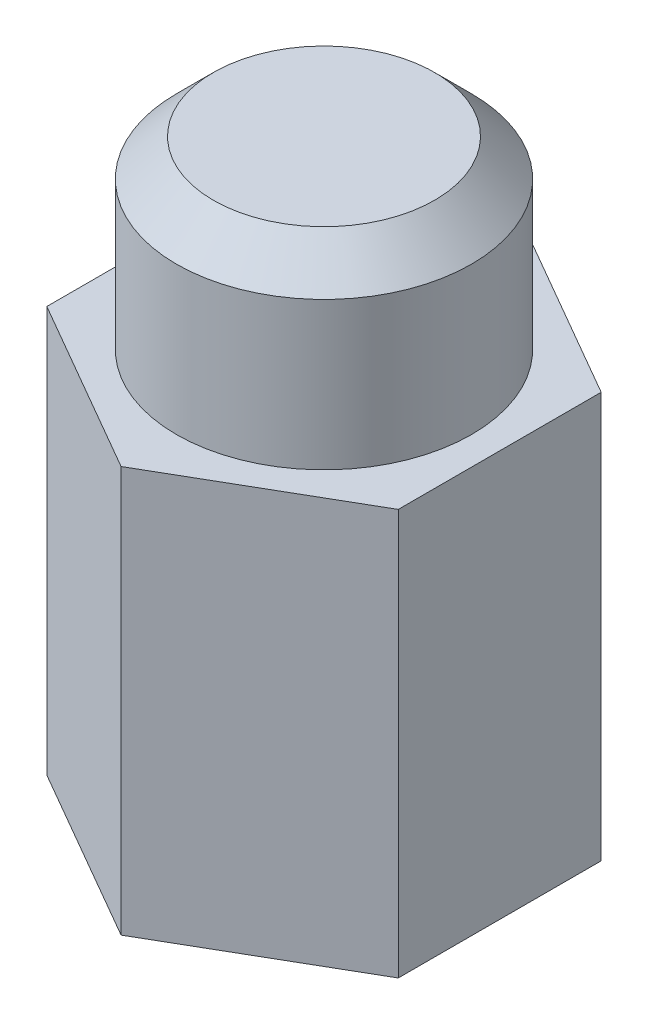
SolidWorks part; units mm, degrees
ref_plane "Front Plane" through (0, 0, 0) normal (0, 0, 1) x (1, 0, 0)
ref_plane "Top Plane" through (0, 0, 0) normal (0, 1, 0) x (1, 0, 0)
ref_plane "Right Plane" through (0, 0, 0) normal (1, 0, 0) x (0, 0, -1)
sketch "Sketch1" plane through (0, 0, 0) normal (0, 1, 0) x (1, 0, 0)
  line L1 (0, 5.5) -> (-4.7631, 2.75)
  line L2 (-4.7631, 2.75) -> (-4.7631, -2.75)
  line L3 (-4.7631, -2.75) -> (0, -5.5)
  line L4 (0, -5.5) -> (4.7631, -2.75)
  line L5 (4.7631, -2.75) -> (4.7631, 2.75)
  line L6 (4.7631, 2.75) -> (0, 5.5)
  circle A0 centre (0, 0) radius 4.7631 construction
  dimension "D1" = 11
extrude "Boss-Extrude1" add sketch "Sketch1" along normal mid plane 11
sketch "Sketch3" plane through (0, 5.5, 0) normal (0, 1, 0) x (1, 0, 0)
  circle A0 centre (0, 0) radius 4
  dimension "D1" = 8
extrude "Boss-Extrude2" add sketch "Sketch3" along normal blind 5
chamfer "Chamfer1" distance 1 angle 45 1 edges at (0, 10.5, 4)
hole_wizard "M6x1.0 Tapped Hole1" positions "Sketch5" profile "Sketch4" tap size "M6x1.0" standard "ANSI Metric"
sketch "Sketch5" plane through (0, -5.5, 0) normal (0, -1, 0) x (-1, 0, 0)
  point P0 (-0.0014, 0)
sketch "Sketch4" plane through (0.0014, -5.5, 0) normal (1, 0, 0) x (0, 0, -1)
  line L0 (0, 0) -> (0, 9.5022)
  line L1 (0, 9.5022) -> (2.5, 8)
  line L2 (2.5, 8) -> (2.5, 0)
  line L5 (2.5, 0) -> (0, 0)
  line L10 (0, 9.5022) -> (-2.5, 8) construction
  line L11 (0, -6.35) -> (0, 107.95) construction
  dimension "Tap Drill Dia." = 5
  dimension "Tap Drill Depth" = 8
  dimension "Drill Angle" = 118
cosmetic thread "Hole Thread1" parameters "D1"=4, "D2"=6
